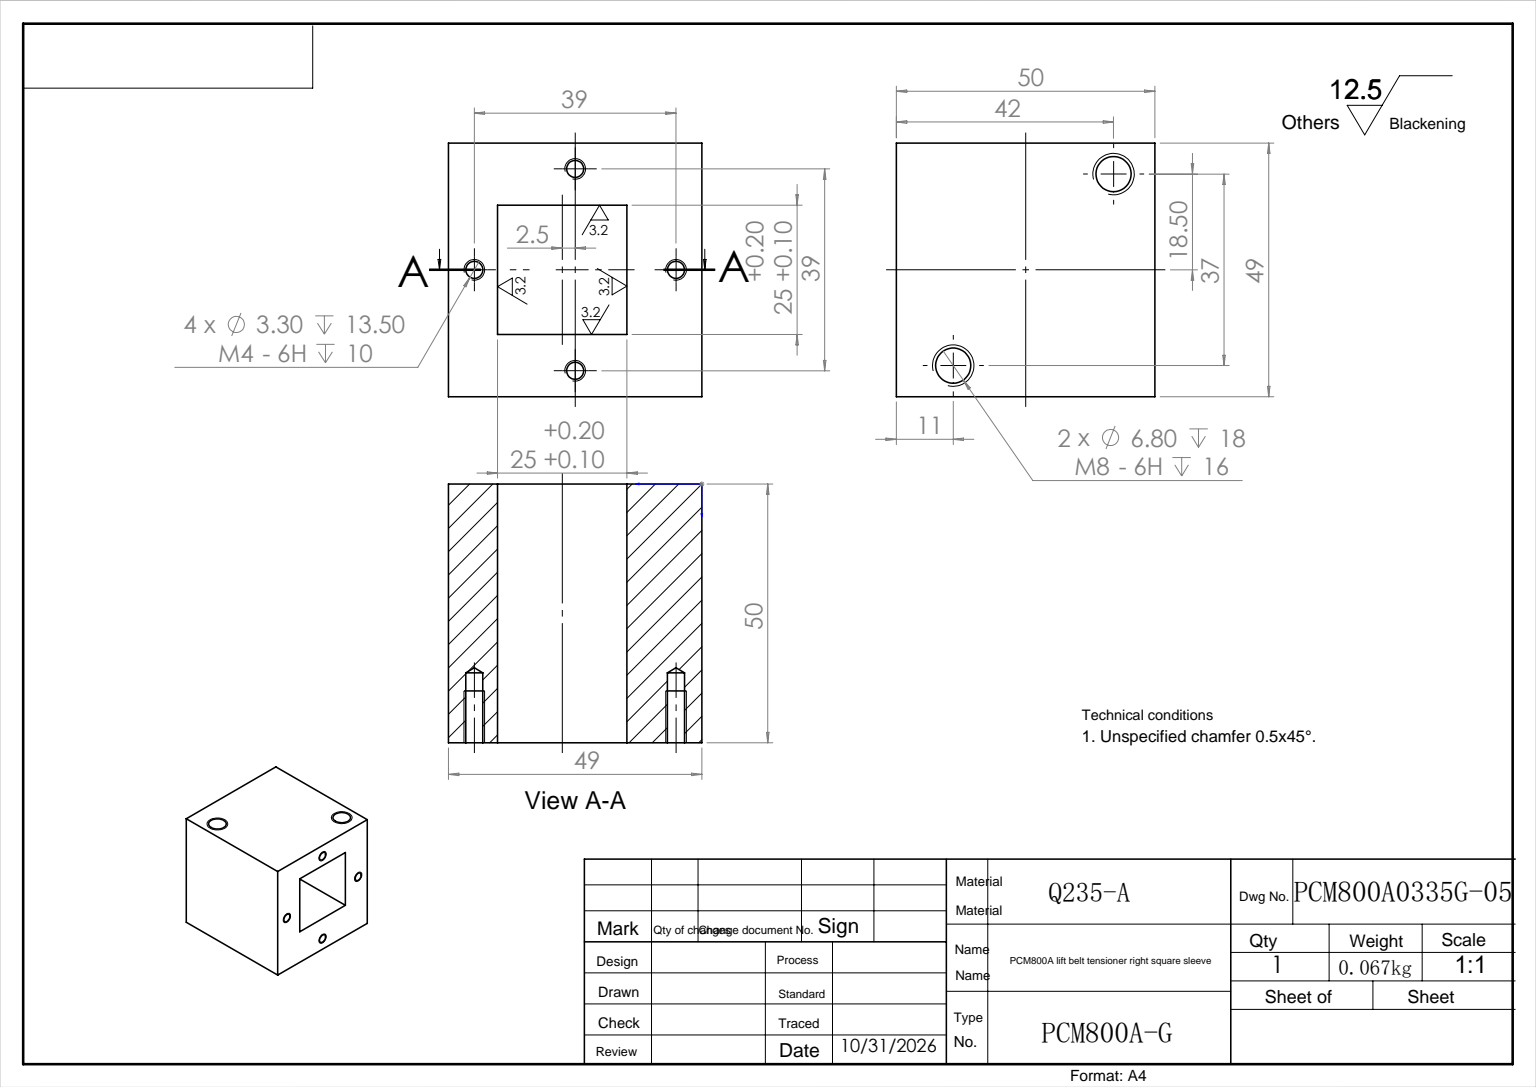
SolidWorks part; units mm, degrees
ref_plane "前视基准面" through (0, 0, 0) normal (0, 0, 1) x (1, 0, 0)
ref_plane "上视基准面" through (0, 0, 0) normal (0, 1, 0) x (1, 0, 0)
ref_plane "右视基准面" through (0, 0, 0) normal (1, 0, 0) x (0, 0, -1)
sketch "草图2" plane through (0, 0, 0) normal (1, 0, 0) x (0, 0, -1)
  line L1 (0, 0) -> (49, 0)
  line L2 (0, 0) -> (0, 49)
  line L3 (0, 49) -> (49, 49)
  line L4 (49, 0) -> (49, 49)
  dimension "D1" = 49
  dimension "D2" = 49
extrude "凸台-拉伸2" add sketch "草图2" along normal blind 50
sketch "草图3" plane through (50, 0, 0) normal (1, 0, 0) x (0, 0, -1)
  line L0 (24.5, 0) -> (24.5, 62.022) construction
  line L1 (12, 39.5) -> (37, 39.5)
  line L2 (12, 39.5) -> (12, 14.5)
  line L3 (12, 14.5) -> (37, 14.5)
  line L4 (37, 39.5) -> (37, 14.5)
  line L5 (0, 0) -> (49, 0) construction
  line L6 (0, 24.5) -> (65.441, 24.5) construction
  line L7 (0, 49) -> (0, 0) construction
  dimension "D1" = 25
  dimension "D2" = 25
  dimension "D3" = 12.5
  dimension "D4" = 15
extrude "切除-拉伸1" cut sketch "草图3" against normal blind 50
hole_wizard "M4 螺纹孔1" positions "草图5" profile "草图4" tap size "M4" standard "GB"
sketch "草图5" plane through (50, 0, 0) normal (1, 0, 0) x (0, 0, -1)
  line L1 (24.5, 49) -> (24.5, -5.0027) construction
  line L2 (49, 49) -> (0, 49) construction
  line L4 (0, 24.5) -> (58.6427, 24.5) construction
  line L5 (0, 49) -> (0, 0) construction
  line L7 (0, 0) -> (49, 0) construction
  line L8 (49, 0) -> (49, 49) construction
  point P0 (24.5, 44)
  point P1 (5, 24.5)
  point P3 (24.5, 5)
  point P5 (44, 24.5)
  dimension "D1" = 5
  dimension "D2" = 5
  dimension "D3" = 5
  dimension "D4" = 5
sketch "草图4" plane through (50, 44, -24.5) normal (0, 1, 0) x (0, 0, -1)
  line L0 (0, 0) -> (0, 14.4914)
  line L1 (0, 14.4914) -> (1.65, 13.5)
  line L2 (1.65, 13.5) -> (1.65, 0)
  line L5 (1.65, 0) -> (0, 0)
  line L10 (0, 14.4914) -> (-1.65, 13.5) construction
  line L11 (0, -6.35) -> (0, 107.95) construction
  dimension "螺纹孔钻头直径" = 3.3
  dimension "螺纹孔钻头深度" = 13.5
  dimension "导头角度" = 118
cosmetic thread "孔螺蚊线1" parameters "D1"=10, "D2"=4
cosmetic thread "孔螺蚊线2" parameters "D1"=10, "D2"=4
cosmetic thread "孔螺蚊线3" parameters "D1"=10, "D2"=4
cosmetic thread "孔螺蚊线4" parameters "D1"=10, "D2"=4
hole_wizard "M8 螺纹孔1" positions "草图7" profile "草图6" tap size "M8" standard "GB"
sketch "草图7" plane through (0, 49, 0) normal (0, 1, 0) x (-1, 0, 0)
  line L0 (0, -49) -> (0, 0) construction
  line L2 (0, -24.5) -> (-61.8244, -24.5) construction
  point P0 (-11, -6)
  point P1 (-42, -43)
  dimension "D1" = 11
  dimension "D2" = 42
  dimension "D3" = 18.5
  dimension "D4" = 18.5
sketch "草图6" plane through (11, 49, -6) normal (1, 0, 0) x (0, 0, 1)
  line L0 (0, 0) -> (0, 20.0429)
  line L1 (0, 20.0429) -> (3.4, 18)
  line L2 (3.4, 18) -> (3.4, 0)
  line L5 (3.4, 0) -> (0, 0)
  line L10 (0, 20.0429) -> (-3.4, 18) construction
  line L11 (0, -6.35) -> (0, 107.95) construction
  dimension "螺纹孔钻头直径" = 6.8
  dimension "螺纹孔钻头深度" = 18
  dimension "导头角度" = 118
cosmetic thread "孔螺蚊线5" parameters "D1"=16, "D2"=8
cosmetic thread "孔螺蚊线6" parameters "D1"=16, "D2"=8
